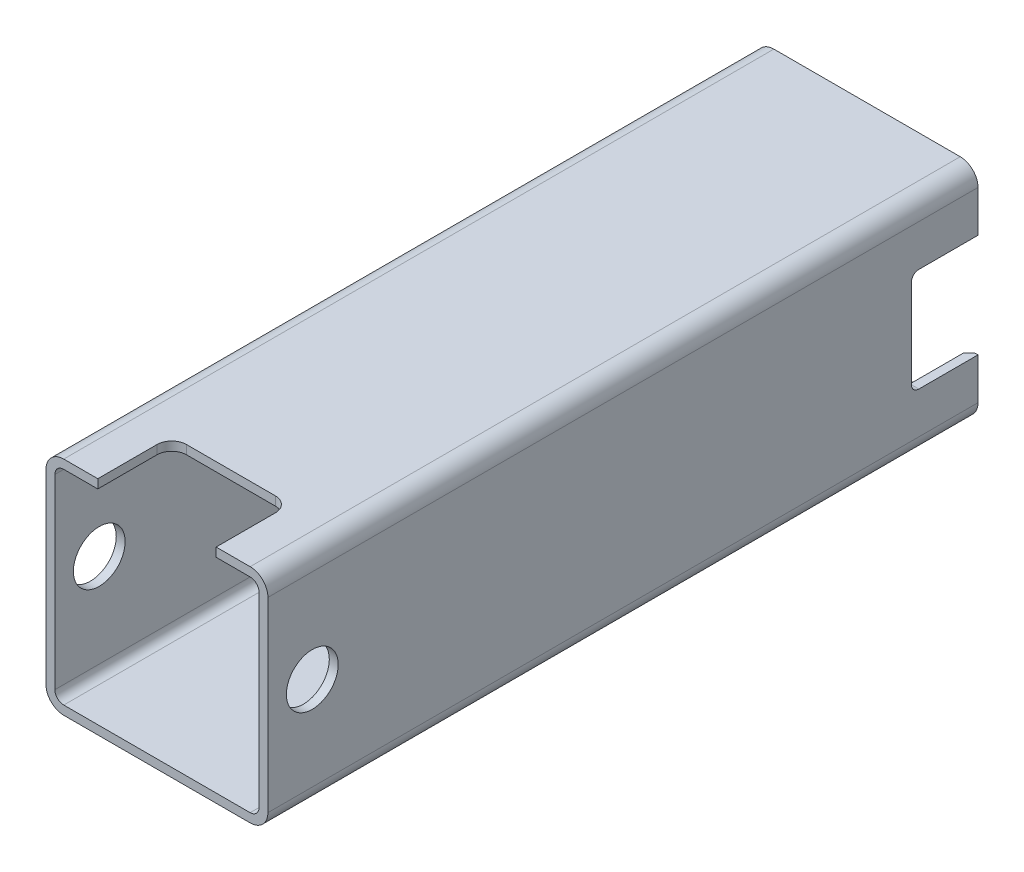
from build123d import *

# Parameters (mm, degrees)
BOSS_EXTRUDE1_DEPTH     = 240
CUT_EXTRUDE1_DEPTH      = 263.392835268
CUT_EXTRUDE2_DEPTH      = 263.392835268
CUT_EXTRUDE2_DEPTH_BACK = 263.392835268
SKETCH2_R               = 17.5
CHAMFER1_SIZE           = 4


with BuildPart() as part:
    # Sketch1 → Boss-Extrude1 (new, symmetric)
    with BuildSketch(Plane.XY):
        with BuildLine():
            Line((-63, -75), (63, -75))
            ThreePointArc((63, -75), (71.485281374, -71.485281374), (75, -63))
            Line((75, -63), (75, 63))
            ThreePointArc((75, 63), (71.485281374, 71.485281374), (63, 75))
            Line((63, 75), (-63, 75))
            ThreePointArc((-63, 75), (-71.485281374, 71.485281374), (-75, 63))
            Line((-75, 63), (-75, -63))
            ThreePointArc((-75, -63), (-71.485281374, -71.485281374), (-63, -75))
        make_face()
        with BuildLine():
            Line((-63, -69), (63, -69))
            ThreePointArc((63, -69), (67.242640687, -67.242640687), (69, -63))
            Line((69, -63), (69, 63))
            ThreePointArc((69, 63), (67.242640687, 67.242640687), (63, 69))
            Line((63, 69), (-63, 69))
            ThreePointArc((-63, 69), (-67.242640687, 67.242640687), (-69, 63))
            Line((-69, 63), (-69, -63))
            ThreePointArc((-69, -63), (-67.242640687, -67.242640687), (-63, -69))
        make_face(mode=Mode.SUBTRACT)
    extrude(amount=BOSS_EXTRUDE1_DEPTH, both=True)

    # 草图1 → Cut-Extrude1 (cut, through all)
    with BuildSketch(Plane(origin=(0, 0, 0), x_dir=(1, 0, 0), z_dir=(0, 1, 0))):
        with BuildLine():
            Line((40, -290), (-40, -290))
            Line((-40, -290), (-40, -200))
            ThreePointArc((-40, -200), (-37.071067812, -192.928932188), (-30, -190))
            Line((-30, -190), (30, -190))
            ThreePointArc((30, -190), (37.071067812, -192.928932188), (40, -200))
            Line((40, -200), (40, -290))
        make_face()
    extrude(amount=CUT_EXTRUDE1_DEPTH, mode=Mode.SUBTRACT)

    # Sketch2 → Cut-Extrude2 (cut, two sides: drawn at the far end of the back side and taken through both)
    with BuildSketch(Plane(origin=(0, 0, 0), x_dir=(0, 0, -1), z_dir=(1, 0, 0)).offset(-CUT_EXTRUDE2_DEPTH_BACK)):
        with Locations((-210, 0)):
            Circle(SKETCH2_R)
        with BuildLine():
            Line((200, 35), (285, 35))
            Line((285, 35), (285, -35))
            Line((285, -35), (200, -35))
            ThreePointArc((200, -35), (196.464466094, -33.535533906), (195, -30))
            Line((195, -30), (195, 30))
            ThreePointArc((195, 30), (196.464466094, 33.535533906), (200, 35))
        make_face()
    extrude(amount=CUT_EXTRUDE2_DEPTH + CUT_EXTRUDE2_DEPTH_BACK, mode=Mode.SUBTRACT)

    # Chamfer1
    chamfer1_edges = [part.edges().sort_by_distance(p)[0] for p in [
        (-67.242640687, 67.242640687, -240),
        (-69, 49, -240),
        (-67.242640687, -67.242640687, -240),
        (0, -69, -240),
        (67.242640687, -67.242640687, -240),
        (69, -49, -240),
        (67.242640687, 67.242640687, -240),
        (0, 69, -240),
        (69, 49, -240),
        (-69, -49, -240),
    ]]
    chamfer(chamfer1_edges, length=CHAMFER1_SIZE)


solid = part.part
